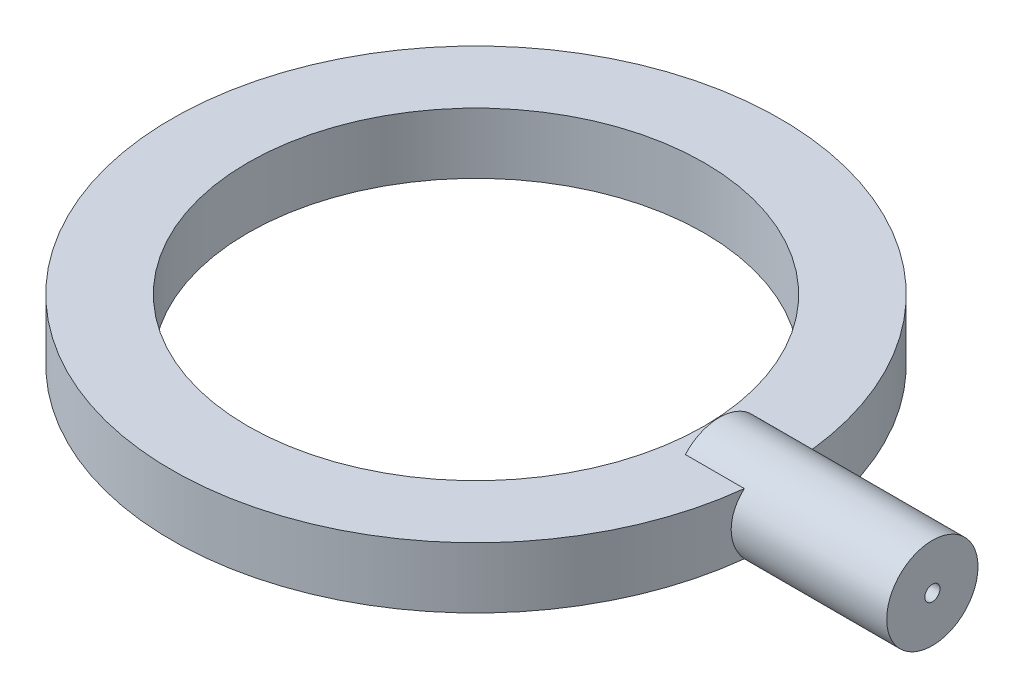
from build123d import *

# Parameters (mm, degrees)
SKETCH1_R             = 100
SKETCH1_R_2           = 75
BOSS_EXTRUDE1_DEPTH   = 20
BOSS_EXTRUDE2_START   = 80
SKETCH2_R             = 15
BOSS_EXTRUDE2_DEPTH   = 70
M6_TAPPED_HOLE1_D     = 5
M6_TAPPED_HOLE1_DEPTH = 17
M6_TAPPED_HOLE1_TIP   = 1.502151548


with BuildPart() as part:
    # Sketch1 → Boss-Extrude1 (new body)
    with BuildSketch(Plane(origin=(0, 0, 0), x_dir=(1, 0, 0), z_dir=(0, 1, 0))):
        with Locations(Location((0, 0, 0), (0, 0, 270))):
            Circle(SKETCH1_R)
        with Locations(Location((0, 0, 0), (0, 0, 270))):
            Circle(SKETCH1_R_2, mode=Mode.SUBTRACT)
    extrude(amount=BOSS_EXTRUDE1_DEPTH)

    # Sketch2 → Boss-Extrude2 (add)
    with BuildSketch(Plane(origin=(0, 0, 0), x_dir=(0, 0, -1), z_dir=(1, 0, 0)).offset(BOSS_EXTRUDE2_START)):
        with Locations(Location((0, 10, 0), (0, 0, 138.189685104))):
            Circle(SKETCH2_R)
    extrude(amount=BOSS_EXTRUDE2_DEPTH)

    # M6 Tapped Hole1
    with Locations(Plane(origin=(150, 0, 0), x_dir=(0, 0, -1), z_dir=(1, 0, 0))):
        with Locations((0, 10)):
            Hole(M6_TAPPED_HOLE1_D / 2, depth=M6_TAPPED_HOLE1_DEPTH)
            with Locations((0, 0, -(M6_TAPPED_HOLE1_DEPTH + M6_TAPPED_HOLE1_TIP / 2))):  # 118° drill point
                Cone(0, M6_TAPPED_HOLE1_D / 2, M6_TAPPED_HOLE1_TIP, mode=Mode.SUBTRACT)


solid = part.part
